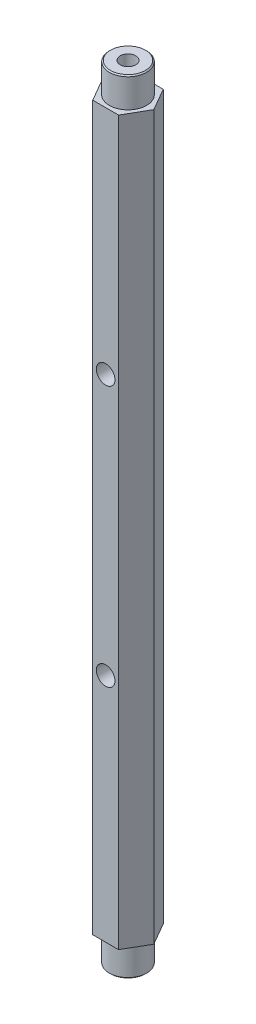
SolidWorks part; units mm, degrees
ref_plane "Front Plane" through (0, 0, 0) normal (0, 0, 1) x (1, 0, 0)
ref_plane "Top Plane" through (0, 0, 0) normal (0, 1, 0) x (1, 0, 0)
ref_plane "Right Plane" through (0, 0, 0) normal (1, 0, 0) x (0, 0, -1)
sketch "Sketch1" plane through (0, 0, 0) normal (0, 1, 0) x (1, 0, 0)
  line L1 (6.9282, 0) -> (3.4641, 6)
  line L2 (3.4641, 6) -> (-3.4641, 6)
  line L3 (-3.4641, 6) -> (-6.9282, 0)
  line L4 (-6.9282, 0) -> (-3.4641, -6)
  line L5 (-3.4641, -6) -> (3.4641, -6)
  line L6 (3.4641, -6) -> (6.9282, 0)
  circle A0 centre (0, 0) radius 6 construction
  dimension "D1" = 12
extrude "Boss-Extrude1" add sketch "Sketch1" along normal blind 210
sketch "Sketch2" plane through (0, 210, 0) normal (0, 1, 0) x (1, 0, 0)
  circle A0 centre (0, 0) radius 5
  dimension "D1" = 10
extrude "Cut-Extrude1" cut sketch "Sketch2" against normal blind 8 flip side to cut
sketch "Sketch3" plane through (0, 0, 0) normal (0, -1, 0) x (1, 0, 0)
  circle A0 centre (0, 0) radius 5
  dimension "D1" = 10
extrude "Cut-Extrude2" cut sketch "Sketch3" against normal blind 8 flip side to cut
hole_wizard "M6 Tapped Hole1" positions "Sketch5" profile "Sketch4" tap size "M6" standard "ISO" end condition through all
sketch "Sketch5" plane through (0, 0, -6) normal (0, 0, -1) x (-1, 0, 0)
  line L0 (3.4641, 202) -> (3.4641, 8) construction
  point P0 (0, 140)
  point P1 (0, 70)
  point P5 (3.4641, 105)
  point P8 (3.4641, 105)
  dimension "D1" = 35
  dimension "D2" = 35
sketch "Sketch4" plane through (0, 140, -6) normal (1, 0, 0) x (0, 1, 0)
  line L0 (0, 0) -> (0, 12)
  line L1 (0, 12) -> (2.5, 12)
  line L2 (2.5, 12) -> (2.5, 0)
  line L5 (2.5, 0) -> (0, 0)
  line L11 (0, -6.35) -> (0, 107.95) construction
  dimension "通孔螺纹孔钻头直径" = 5
  dimension "通孔螺纹孔钻头深度" = 12
cosmetic thread "Cosmetic Thread1" parameters "D2"=6
cosmetic thread "Cosmetic Thread2" parameters "D2"=6
hole_wizard "M5 Tapped Hole1" positions "Sketch7" profile "Sketch6" tap size "M5" standard "ISO"
sketch "Sketch7" plane through (0, 0, 0) normal (0, -1, 0) x (1, 0, 0)
  point P0 (0, 0)
sketch "Sketch6" plane through (0, 0, 0) normal (1, 0, 0) x (0, 0, -1)
  line L0 (0, 0) -> (0, 13.6618)
  line L1 (0, 13.6618) -> (2.1, 12.4)
  line L2 (2.1, 12.4) -> (2.1, 0)
  line L5 (2.1, 0) -> (0, 0)
  line L10 (0, 13.6618) -> (-2.1, 12.4) construction
  line L11 (0, -6.35) -> (0, 107.95) construction
  dimension "螺纹孔钻头直径" = 4.2
  dimension "螺纹孔钻头深度" = 12.4
  dimension "导头角度" = 118
cosmetic thread "Cosmetic Thread3" parameters "D1"=10, "D2"=5
hole_wizard "M5 Tapped Hole2" positions "Sketch9" profile "Sketch8" tap size "M5" standard "ISO"
sketch "Sketch9" plane through (0, 210, 0) normal (0, 1, 0) x (-1, 0, 0)
  point P0 (0, 0)
sketch "Sketch8" plane through (0, 210, 0) normal (1, 0, 0) x (0, 0, 1)
  line L0 (0, 0) -> (0, 13.6618)
  line L1 (0, 13.6618) -> (2.1, 12.4)
  line L2 (2.1, 12.4) -> (2.1, 0)
  line L5 (2.1, 0) -> (0, 0)
  line L10 (0, 13.6618) -> (-2.1, 12.4) construction
  line L11 (0, -6.35) -> (0, 107.95) construction
  dimension "螺纹孔钻头直径" = 4.2
  dimension "螺纹孔钻头深度" = 12.4
  dimension "导头角度" = 118
cosmetic thread "Cosmetic Thread4" parameters "D1"=10, "D2"=5
chamfer "Chamfer1" distance 0.3 angle 45 2 edges at (0, 0, -5) (0, 210, 5)
